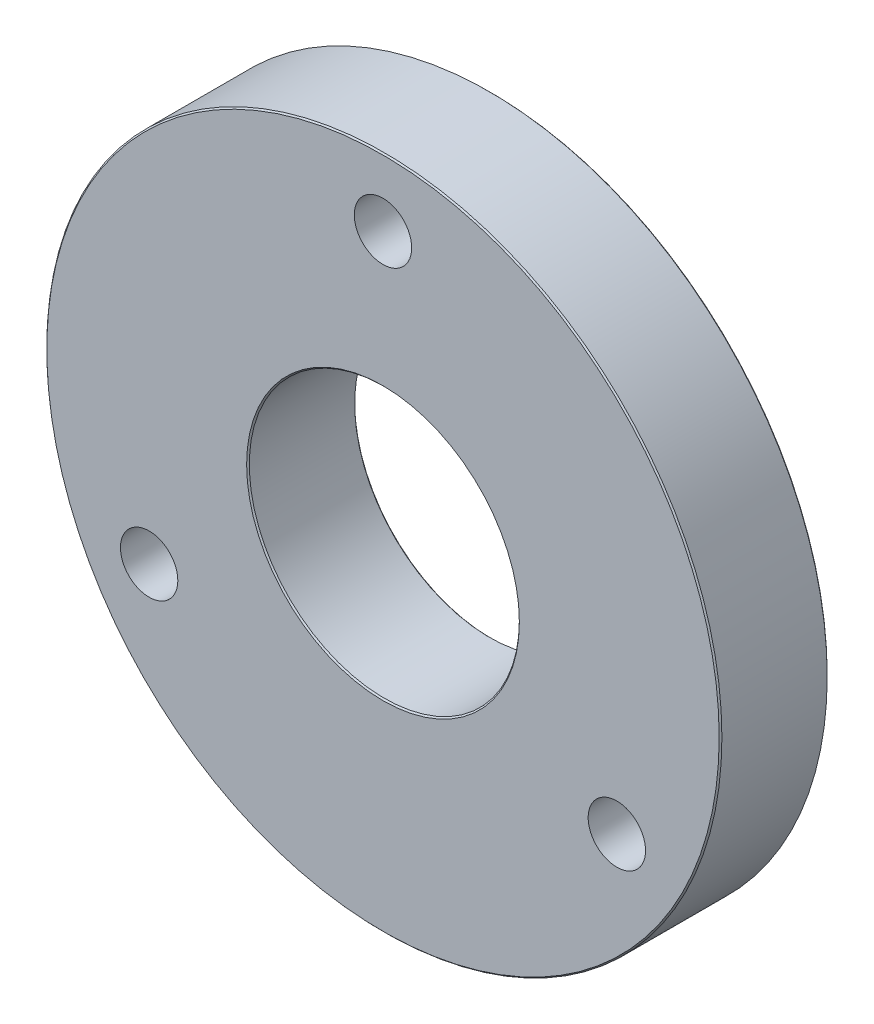
SolidWorks part; units mm, degrees
material "Q235"
ref_plane "Front Plane" through (0, 0, 0) normal (0, 0, 1) x (1, 0, 0)
ref_plane "Top Plane" through (0, 0, 0) normal (0, 1, 0) x (1, 0, 0)
ref_plane "Right Plane" through (0, 0, 0) normal (1, 0, 0) x (0, 0, -1)
sketch "Sketch1" plane through (0, 0, 0) normal (0, 0, 1) x (1, 0, 0)
  circle A0 centre (0, 0) radius 50
  circle A1 centre (0, 0) radius 20
  dimension "D1" = 100
  dimension "D2" = 40
extrude "Boss-Extrude1" add sketch "Sketch1" along normal blind 16
hole_wizard "M10 Tapped Hole1" positions "Sketch4" profile "Sketch5" tap size "M10" standard "GB"
sketch "Sketch4" plane through (0, 0, 16) normal (0, 0, 1) x (1, 0, 0)
  line L0 (0, 0) -> (0, 40) construction
  point P0 (0, 40)
  dimension "D1" = 40
sketch "Sketch5" plane through (0, 40, 16) normal (1, 0, 0) x (0, -1, 0)
  line L0 (0, 0) -> (0, 31.8037)
  line L1 (0, 31.8037) -> (4.25, 29.25)
  line L2 (4.25, 29.25) -> (4.25, 0)
  line L5 (4.25, 0) -> (0, 0)
  line L10 (0, 31.8037) -> (-4.25, 29.25) construction
  line L11 (0, -6.35) -> (0, 107.95) construction
  dimension "螺纹孔钻头直径" = 8.5
  dimension "螺纹孔钻头深度" = 29.25
  dimension "导头角度" = 118
cosmetic thread "Cosmetic Thread1"
pattern_circular "CirPattern1" count 3 every 120 about axis through (0, 0, 0) along (0, 0, 1) of "M10 Tapped Hole1"
cosmetic thread "Cosmetic Thread2"
cosmetic thread "Cosmetic Thread3"
cosmetic thread "Cosmetic Thread4"
cosmetic thread "Cosmetic Thread5"
cosmetic thread "Cosmetic Thread6"
chamfer "Chamfer1" distance 0.2 angle 45 4 edges at (20, 0, 16) (20, 0, 0) (50, 0, 0) (50, 0, 16)
